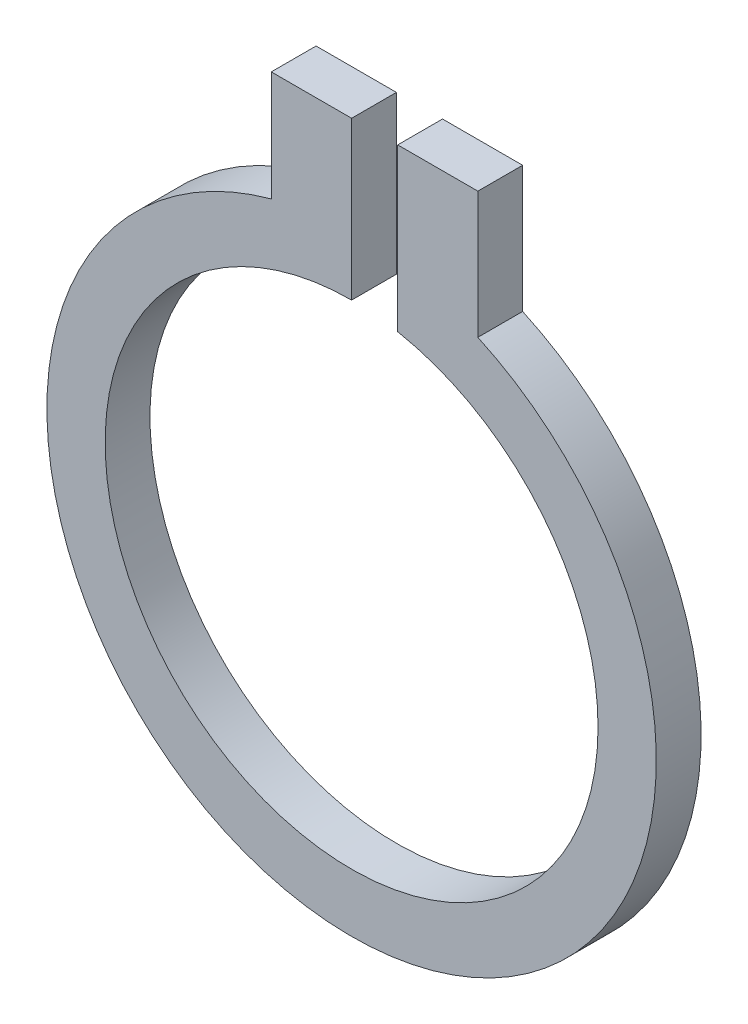
from build123d import *

# Parameters (mm, degrees)
BOSS_EXTRUDE1_DEPTH = 1


with BuildPart() as part:
    # Sketch1 → Boss-Extrude1 (new body)
    with BuildSketch(Plane.XY):
        with BuildLine():
            Line((1.029116593, 5.402862115), (1.029116593, 9.014895643))
            Line((1.029116593, 9.014895643), (2.817154888, 9.014895643))
            Line((2.817154888, 9.014895643), (2.817154888, 6.188993322))
            ThreePointArc((2.817154888, 6.188993322), (-0.544669265, -6.778151326), (-1.792734929, 6.559428441))
            Line((-1.792734929, 6.559428441), (-1.792734929, 9.014895643))
            Line((-1.792734929, 9.014895643), (0, 9.014895643))
            Line((0, 9.014895643), (0, 5.5))
            ThreePointArc((0, 5.5), (-0.516845415, -5.475661678), (1.029116593, 5.402862115))
        make_face()
    extrude(amount=BOSS_EXTRUDE1_DEPTH)


solid = part.part
